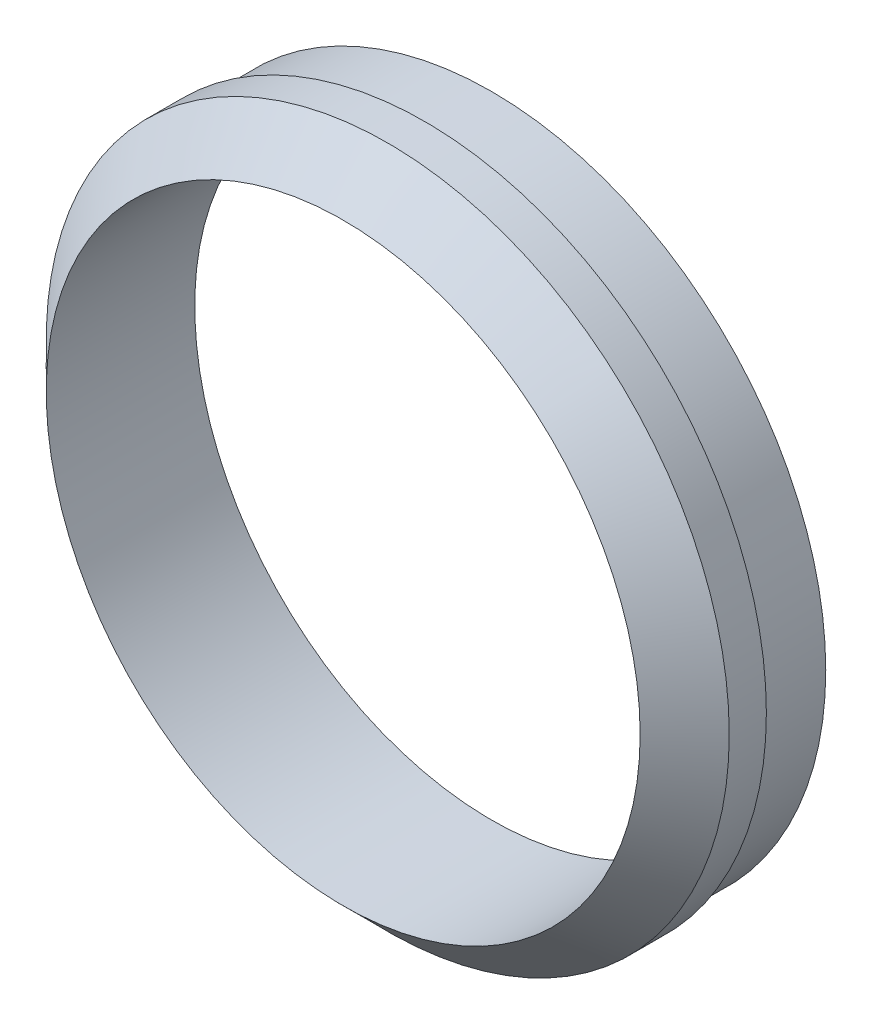
SolidWorks part; units mm, degrees
ref_plane "Front Plane" through (0, 0, 0) normal (0, 0, 1) x (1, 0, 0)
ref_plane "Top Plane" through (0, 0, 0) normal (0, 1, 0) x (1, 0, 0)
ref_plane "Right Plane" through (0, 0, 0) normal (1, 0, 0) x (0, 0, -1)
other "Configuration Table"
sketch "Sketch1" plane through (0, 0, 0) normal (0, 1, 0) x (1, 0, 0)
  line L0 (8, 4) -> (8, 0)
  line L1 (8, 0) -> (9.2, 1.2)
  line L2 (9.2, 1.2) -> (9.2, 2.2)
  line L3 (9.2, 2.2) -> (9, 2.2)
  line L4 (9, 2.2) -> (9, 4)
  line L5 (9, 4) -> (8, 4)
  line L6 (0, 4) -> (0, 0) construction
revolve "Revolve1" add sketch "Sketch1" angle 360 about L6
